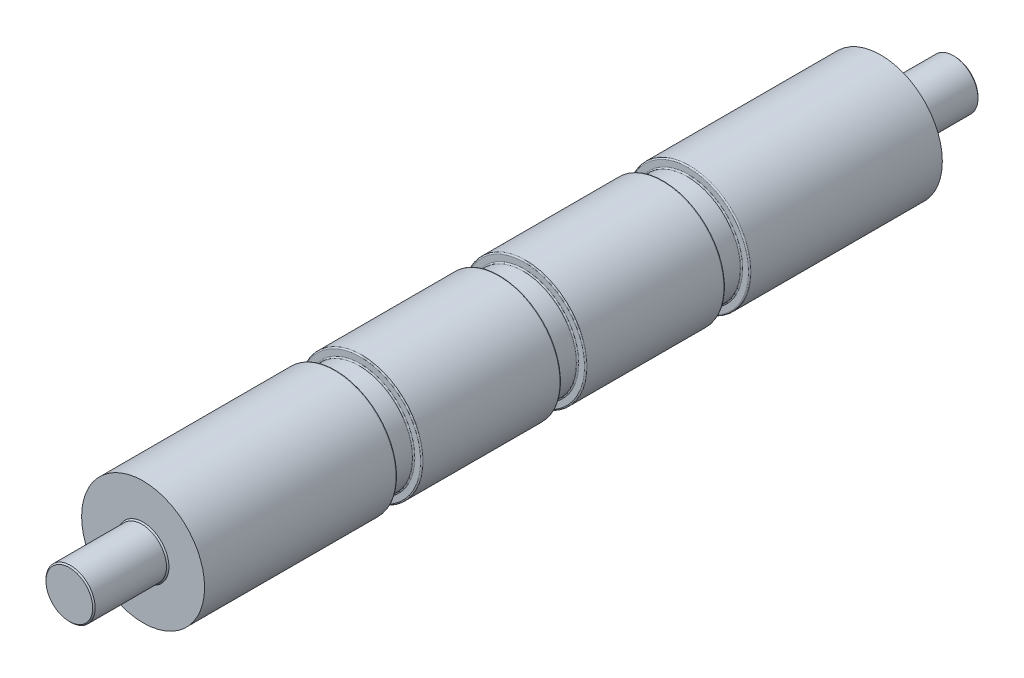
from build123d import *

# Parameters (mm, degrees)
SKETCH1_R                  = 150
BOSS_EXTRUDE1_DEPTH        = 1800
SKETCH2_W                  = 40
SKETCH2_H                  = 60
FILLET1_R                  = 3
LPATTERN1_COUNT            = 2
LPATTERN1_PITCH            = 400
FILLET1_OF_LPATTERN1_R     = 3
LPATTERN1_COL_COUNT        = 2
LPATTERN1_COL_PITCH        = 400
FILLET1_OF_LPATTERN1_COL_R = 3
SKETCH3_R                  = 60
BOSS_EXTRUDE2_DEPTH        = 180
CHAMFER1_SIZE              = 3
BOSS_EXTRUDE3_START        = 180
SKETCH4_R                  = 60
BOSS_EXTRUDE3_DEPTH        = 180
CHAMFER2_SIZE              = 3


with BuildPart() as part:
    # Sketch1 → Boss-Extrude1 (new body)
    with BuildSketch(Plane.XY):
        Circle(SKETCH1_R)
    extrude(amount=BOSS_EXTRUDE1_DEPTH)

    # Sketch2 → Cut-Revolve1 (revolve, cut)
    with BuildSketch(Plane(origin=(0, 0, 0), x_dir=(1, 0, 0), z_dir=(0, 1, 0)), mode=Mode.PRIVATE) as cut_revolve1_sk:
        with Locations((150, -900)):
            Rectangle(SKETCH2_W, SKETCH2_H)
    cut_revolve1 = revolve(cut_revolve1_sk.sketch.rotate(Axis((0, 0, 0), (0, 0, 1)), 180), axis=Axis((0, 0, 0), (0, 0, 1)), mode=Mode.SUBTRACT)

    # Fillet1
    fillet1_edges = [part.edges().sort_by_distance(p)[0] for p in [
        (130, 0, 930),
        (-150, 0, 930),
        (130, 0, 870),
        (-150, 0, 870),
    ]]
    fillet(fillet1_edges, radius=FILLET1_R)

    # LPattern1: Cut-Revolve1 ×2
    with Locations(*[(0, 0, -i * LPATTERN1_PITCH) for i in range(1, LPATTERN1_COUNT)]):
        add(cut_revolve1, mode=Mode.SUBTRACT)

    # Fillet1 of LPattern1
    fillet1_of_lpattern1_edges = [part.edges().sort_by_distance(p)[0] for p in [
        (130, 0, 530),
        (-150, 0, 530),
        (130, 0, 470),
        (-150, 0, 470),
    ]]
    fillet(fillet1_of_lpattern1_edges, radius=FILLET1_OF_LPATTERN1_R)

    # LPattern1 col: Cut-Revolve1 ×2
    with Locations(*[(0, 0, i * LPATTERN1_COL_PITCH) for i in range(1, LPATTERN1_COL_COUNT)]):
        add(cut_revolve1, mode=Mode.SUBTRACT)

    # Fillet1 of LPattern1 col
    fillet1_of_lpattern1_col_edges = [part.edges().sort_by_distance(p)[0] for p in [
        (130, 0, 1330),
        (-150, 0, 1330),
        (130, 0, 1270),
        (-150, 0, 1270),
    ]]
    fillet(fillet1_of_lpattern1_col_edges, radius=FILLET1_OF_LPATTERN1_COL_R)

    # Sketch3 → Boss-Extrude2 (add)
    with BuildSketch(Plane.XY.offset(1800)):
        Circle(SKETCH3_R)
    extrude(amount=BOSS_EXTRUDE2_DEPTH)

    # Chamfer1
    chamfer1_edges = [part.edges().sort_by_distance(p)[0] for p in [
        (-60, 0, 1800),
        (-60, 0, 1980),
    ]]
    chamfer(chamfer1_edges, length=CHAMFER1_SIZE)

    # Sketch4 → Boss-Extrude3 (add)
    with BuildSketch(Plane(origin=(0, 0, 0), x_dir=(-1, 0, 0), z_dir=(0, 0, -1)).offset(BOSS_EXTRUDE3_START)):
        with Locations(Location((0, 0, 0), (0, 0, 180))):
            Circle(SKETCH4_R)
    extrude(amount=-BOSS_EXTRUDE3_DEPTH)

    # Chamfer2
    chamfer2_edges = [part.edges().sort_by_distance(p)[0] for p in [
        (-60, 0, 0),
        (-60, 0, -180),
    ]]
    chamfer(chamfer2_edges, length=CHAMFER2_SIZE)


solid = part.part
